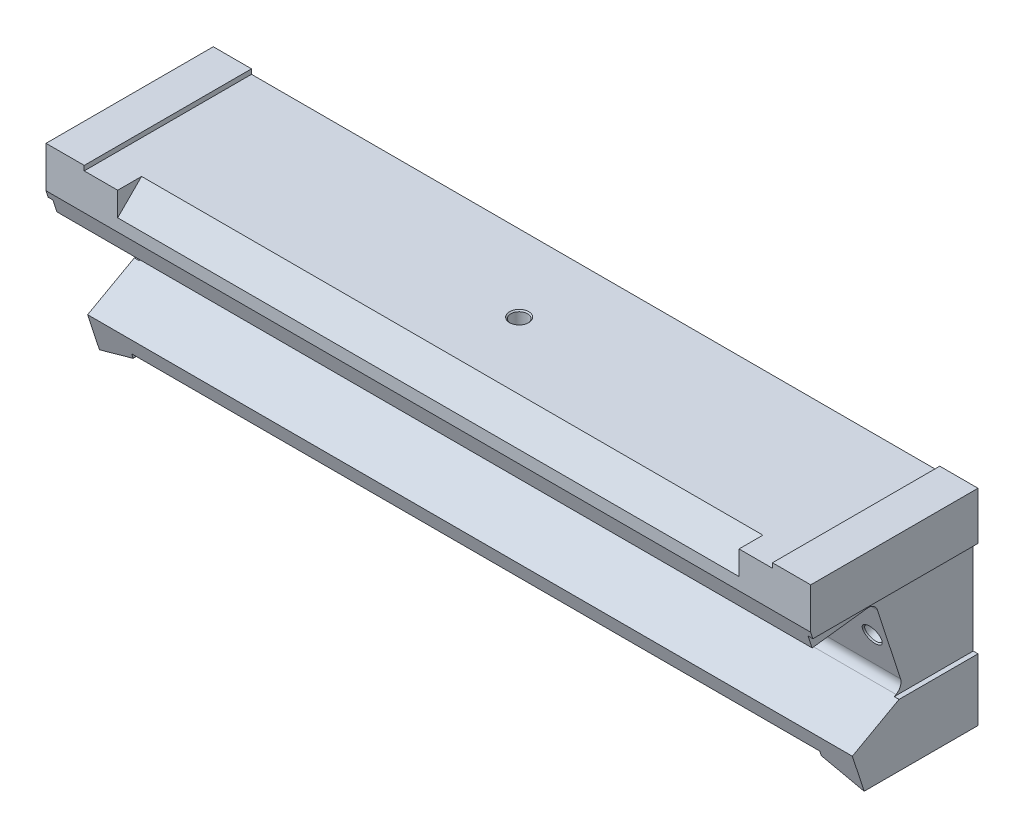
from build123d import *

# Parameters (mm, degrees)
BOSS_EXTRUDE1_DEPTH                    = 400
SKETCH3_W                              = 720
SKETCH3_H                              = 10
CUT_EXTRUDE1_DEPTH                     = 487.672374396
CUT_EXTRUDE2_DEPTH                     = 325
CUT_EXTRUDE3_DEPTH                     = 650
SKETCH7_W                              = 10
SKETCH7_H                              = 100
CUT_EXTRUDE4_DEPTH                     = 650
BOSS_EXTRUDE2_REACH                    = 488.672
SKETCH8_W                              = 40
SKETCH8_H                              = 100
SKETCH8_W_2                            = 35
M20_TAPPED_HOLE1_D                     = 17.5
M20_TAPPED_HOLE1_DEPTH                 = 45
M20_TAPPED_HOLE1_CSINK_D               = 20.05
M20_TAPPED_HOLE1_CSINK_ANGLE           = 90
M20_TAPPED_HOLE1_TIP                   = 5.257530416
M20_TAPPED_HOLE2_D                     = 17.5
M20_TAPPED_HOLE2_DEPTH                 = 40
M20_TAPPED_HOLE2_CSINK_D               = 20.05
M20_TAPPED_HOLE2_CSINK_ANGLE           = 90
M20_TAPPED_HOLE2_TIP                   = 5.257530416
M20_TAPPED_HOLE2_ON_FACE_2_D           = 17.5
M20_TAPPED_HOLE2_ON_FACE_2_DEPTH       = 40
M20_TAPPED_HOLE2_ON_FACE_2_CSINK_D     = 20.05
M20_TAPPED_HOLE2_ON_FACE_2_CSINK_ANGLE = 90
M20_TAPPED_HOLE2_ON_FACE_2_TIP         = 5.257530416
FILLET1_R                              = 10


with BuildPart() as part:
    # Sketch1 → Boss-Extrude1 (new, symmetric)
    with BuildSketch(Plane(origin=(0, 0, 0), x_dir=(0, 0, -1), z_dir=(1, 0, 0))):
        Polygon((0, 0), (-119.1, 0), (-131.429467258, 37.946198403), (-73.515136927, 70.048635914), (-102.788489796, 160.142752116), (-168.511506583, 152.072980358), (-175, 172.042509728), (-175, 215), (0, 215), (0, 165), (-51.793594091, 165), (-19.301624468, 65), (0, 65), align=None)
    extrude(amount=BOSS_EXTRUDE1_DEPTH, both=True)

    # Sketch3 → Cut-Extrude1 (cut, through all)
    with BuildSketch(Plane.XY):
        with Locations((0, 215)):
            Rectangle(SKETCH3_W, SKETCH3_H)
    extrude(amount=CUT_EXTRUDE1_DEPTH, mode=Mode.SUBTRACT)

    # Sketch4 → Cut-Extrude2 (cut, symmetric)
    with BuildSketch(Plane(origin=(0, 0, 0), x_dir=(0, 0, -1), z_dir=(1, 0, 0))):
        Polygon((-175, 215), (-175, 185), (-145, 215), align=None)
    extrude(amount=CUT_EXTRUDE2_DEPTH, both=True, mode=Mode.SUBTRACT)

    # Sketch6 → Cut-Extrude3 (cut)
    with BuildSketch(Plane(origin=(0, 0, 0), x_dir=(-1, 0, 0), z_dir=(0, 0, -1))):
        Polygon((-400, 0), (-360, 14.558809371), (-360, 19.558809371), (360, 19.558809371), (360, 14.558809371), (400, 0), align=None)
    extrude(amount=-CUT_EXTRUDE3_DEPTH, mode=Mode.SUBTRACT)

    # Sketch7 → Cut-Extrude4 (cut)
    with BuildSketch(Plane.XY):
        with Locations((-400, 115)):
            Rectangle(SKETCH7_W, SKETCH7_H)
    cut_extrude4 = extrude(amount=CUT_EXTRUDE4_DEPTH, mode=Mode.SUBTRACT)

    # Mirror1: Cut-Extrude4 across plane
    add(cut_extrude4.mirror(Plane(origin=(0, 0, 0), x_dir=(0, 0, 1), z_dir=(1, 0, 0))), mode=Mode.SUBTRACT)

    # Boss-Extrude2: up to this plane
    boss_extrude2_end = Plane(origin=(400, 165, 51.793594091), z_dir=(0, -0.309016994374942, 0.9510565162951553))
    # Sketch8 → Boss-Extrude2 (add, up to the surface)
    with BuildSketch(Plane(origin=(0, 0, 0), x_dir=(-1, 0, 0), z_dir=(0, 0, -1)), mode=Mode.PRIVATE) as boss_extrude2_sk1:
        with Locations((0, 115)):
            Rectangle(SKETCH8_W, SKETCH8_H)
    boss_extrude2_tool1 = split(extrude(boss_extrude2_sk1.sketch, amount=-BOSS_EXTRUDE2_REACH, mode=Mode.PRIVATE), bisect_by=boss_extrude2_end, keep=Keep.BOTH, mode=Mode.PRIVATE)
    add(boss_extrude2_tool1.solids().sort_by_distance((0, 115, 0))[0])
    # Sketch8 → Boss-Extrude2 (add, up to the surface)
    with BuildSketch(Plane(origin=(0, 0, 0), x_dir=(-1, 0, 0), z_dir=(0, 0, -1)), mode=Mode.PRIVATE) as boss_extrude2_sk2:
        with Locations((-190, 115)):
            Rectangle(SKETCH8_W, SKETCH8_H)
    boss_extrude2_tool2 = split(extrude(boss_extrude2_sk2.sketch, amount=-BOSS_EXTRUDE2_REACH, mode=Mode.PRIVATE), bisect_by=boss_extrude2_end, keep=Keep.BOTH, mode=Mode.PRIVATE)
    add(boss_extrude2_tool2.solids().sort_by_distance((190, 115, 0))[0])
    # Sketch8 → Boss-Extrude2 (add, up to the surface)
    with BuildSketch(Plane(origin=(0, 0, 0), x_dir=(-1, 0, 0), z_dir=(0, 0, -1)), mode=Mode.PRIVATE) as boss_extrude2_sk3:
        with Locations((190, 115)):
            Rectangle(SKETCH8_W, SKETCH8_H)
    boss_extrude2_tool3 = split(extrude(boss_extrude2_sk3.sketch, amount=-BOSS_EXTRUDE2_REACH, mode=Mode.PRIVATE), bisect_by=boss_extrude2_end, keep=Keep.BOTH, mode=Mode.PRIVATE)
    add(boss_extrude2_tool3.solids().sort_by_distance((-190, 115, 0))[0])
    # Sketch8 → Boss-Extrude2 (add, up to the surface)
    with BuildSketch(Plane(origin=(0, 0, 0), x_dir=(-1, 0, 0), z_dir=(0, 0, -1)), mode=Mode.PRIVATE) as boss_extrude2_sk4:
        with Locations((-377.5, 115)):
            Rectangle(SKETCH8_W_2, SKETCH8_H)
    boss_extrude2_tool4 = split(extrude(boss_extrude2_sk4.sketch, amount=-BOSS_EXTRUDE2_REACH, mode=Mode.PRIVATE), bisect_by=boss_extrude2_end, keep=Keep.BOTH, mode=Mode.PRIVATE)
    add(boss_extrude2_tool4.solids().sort_by_distance((377.5, 115, 0))[0])
    # Sketch8 → Boss-Extrude2 (add, up to the surface)
    with BuildSketch(Plane(origin=(0, 0, 0), x_dir=(-1, 0, 0), z_dir=(0, 0, -1)), mode=Mode.PRIVATE) as boss_extrude2_sk5:
        with Locations((377.5, 115)):
            Rectangle(SKETCH8_W_2, SKETCH8_H)
    boss_extrude2_tool5 = split(extrude(boss_extrude2_sk5.sketch, amount=-BOSS_EXTRUDE2_REACH, mode=Mode.PRIVATE), bisect_by=boss_extrude2_end, keep=Keep.BOTH, mode=Mode.PRIVATE)
    add(boss_extrude2_tool5.solids().sort_by_distance((-377.5, 115, 0))[0])

    # M20 Tapped Hole1
    with Locations(Plane(origin=(0, 210, 80), x_dir=(0, 0, 1), z_dir=(0, 1, 0))):
        with Locations((0, 0)):
            CounterSinkHole(M20_TAPPED_HOLE1_D / 2, M20_TAPPED_HOLE1_CSINK_D / 2, depth=M20_TAPPED_HOLE1_DEPTH, counter_sink_angle=M20_TAPPED_HOLE1_CSINK_ANGLE)
            with Locations((0, 0, -(M20_TAPPED_HOLE1_DEPTH + M20_TAPPED_HOLE1_TIP / 2))):  # 118° drill point
                Cone(0, M20_TAPPED_HOLE1_D / 2, M20_TAPPED_HOLE1_TIP, mode=Mode.SUBTRACT)

    # M20 Tapped Hole2
    with Locations(Plane(origin=(-377.5, 115.095694015, 88.151813362), x_dir=(0, 0.951056516295, 0.309016994375), z_dir=(0, -0.309016994375, 0.951056516295))):
        with Locations((0, 0)):
            CounterSinkHole(M20_TAPPED_HOLE2_D / 2, M20_TAPPED_HOLE2_CSINK_D / 2, depth=M20_TAPPED_HOLE2_DEPTH, counter_sink_angle=M20_TAPPED_HOLE2_CSINK_ANGLE)
            with Locations((0, 0, -(M20_TAPPED_HOLE2_DEPTH + M20_TAPPED_HOLE2_TIP / 2))):  # 118° drill point
                Cone(0, M20_TAPPED_HOLE2_D / 2, M20_TAPPED_HOLE2_TIP, mode=Mode.SUBTRACT)

    # M20 Tapped Hole2 on face 2
    with Locations(Plane(origin=(0, 115.095694015, 88.151813362), x_dir=(0, 0.951056560832, 0.309016857306), z_dir=(0, -0.309016857306, 0.951056560832))):
        with Locations((0, 0), (0, -377.5)):
            CounterSinkHole(M20_TAPPED_HOLE2_ON_FACE_2_D / 2, M20_TAPPED_HOLE2_ON_FACE_2_CSINK_D / 2, depth=M20_TAPPED_HOLE2_ON_FACE_2_DEPTH, counter_sink_angle=M20_TAPPED_HOLE2_ON_FACE_2_CSINK_ANGLE)
            with Locations((0, 0, -(M20_TAPPED_HOLE2_ON_FACE_2_DEPTH + M20_TAPPED_HOLE2_ON_FACE_2_TIP / 2))):  # 118° drill point
                Cone(0, M20_TAPPED_HOLE2_ON_FACE_2_D / 2, M20_TAPPED_HOLE2_ON_FACE_2_TIP, mode=Mode.SUBTRACT)

    # Fillet1
    fillet1_edges = [part.edges().sort_by_distance(p)[0] for p in [
        (0, 70.048635914, 73.515136927),
        (0, 160.142752116, 102.788489796),
    ]]
    fillet(fillet1_edges, radius=FILLET1_R)


solid = part.part
